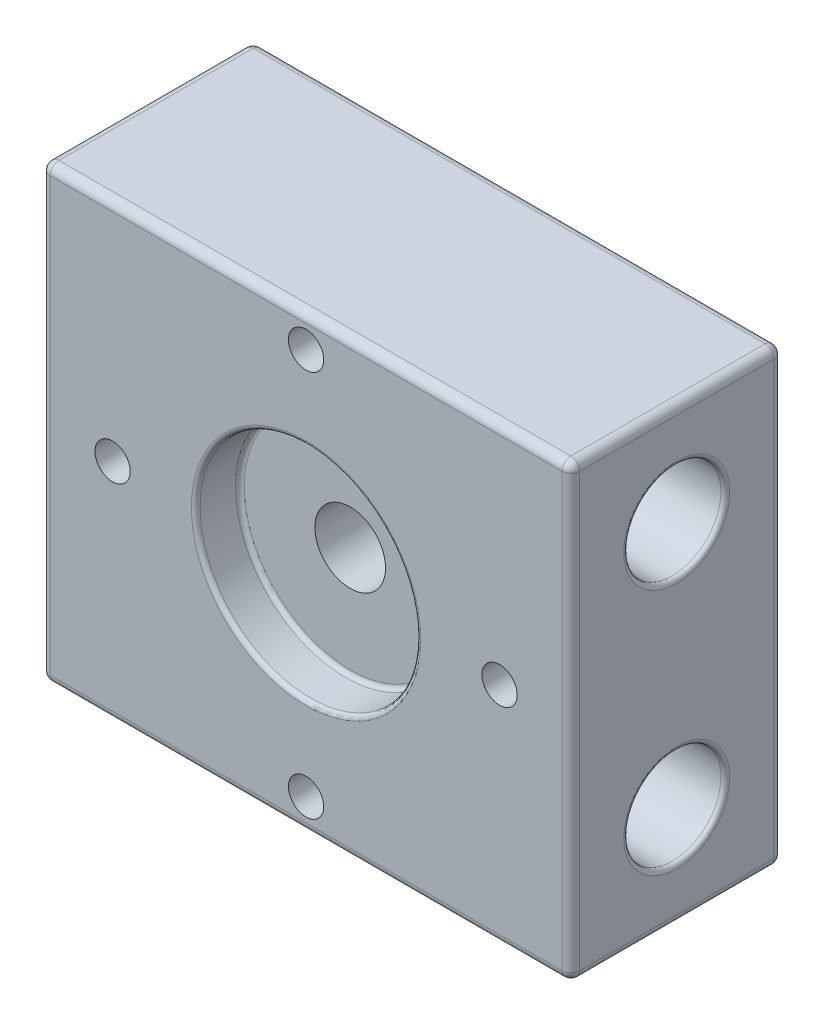
SolidWorks part; units mm, degrees
material "ABS PC"
ref_plane "Front Plane" through (0, 0, 0) normal (0, 0, 1) x (1, 0, 0)
ref_plane "Top Plane" through (0, 0, 0) normal (0, 1, 0) x (1, 0, 0)
ref_plane "Right Plane" through (0, 0, 0) normal (1, 0, 0) x (0, 0, -1)
sketch "Sketch1" plane through (0, 0, 0) normal (0, 0, 1) x (1, 0, 0)
  line L1 (30, -25.5) -> (-30, -25.5)
  line L2 (30, -25.5) -> (30, 25.5)
  line L3 (30, 25.5) -> (-30, 25.5)
  line L4 (-30, -25.5) -> (-30, 25.5)
  line L5 (30, -25.5) -> (-30, 25.5) construction
  line L6 (30, 25.5) -> (-30, -25.5) construction
  point P0 (0, 0)
  dimension "D1" = 60
  dimension "D2" = 51
extrude "Boss-Extrude1" add sketch "Sketch1" along normal mid plane 24
sketch "Sketch2" plane through (0, 0, 12) normal (0, 0, 1) x (1, 0, 0)
  circle A0 centre (0, 0) radius 12.5
  dimension "D1" = 25
extrude "Cut-Extrude1" cut sketch "Sketch2" against normal blind 5
sketch "Sketch3" plane through (30, 0, 0) normal (1, 0, 0) x (0, 0, -1)
  line L0 (0, 0) -> (17.8239, 0) construction
  circle A0 centre (0, 14) radius 5.5
  circle A1 centre (0, -14) radius 5.5
  dimension "D1" = 28
  dimension "D2" = 11
extrude "Cut-Extrude2" cut sketch "Sketch3" against normal through all
fillet "Fillet1" radius 1 12 edges at (-30, -25.5, 0) (0, -25.5, 12) (30, -25.5, 0) (0, -25.5, -12) (30, 25.5, 0) (0, 25.5, 12) (-30, 25.5, 0) (0, 25.5, -12) (-30, 0, -12) (30, 0, -12) (-30, 0, 12) (30, 0, 12)
fillet "Fillet2" radius 0.5 6 edges at (12.5, 0, 12) (12.5, 0, 7) (30, -14, -5.5) (-30, -14, -5.5) (30, 14, -5.5) (-30, 14, -5.5)
sketch "Sketch4" plane through (0, 0, -12) normal (0, 0, -1) x (-1, 0, 0)
  circle A0 centre (0, 0) radius 12.5
  circle A1 centre (0, 0) radius 4
  circle A2 centre (0, 0) radius 12 construction
  dimension "D1" = 25
  dimension "D2" = 8
extrude "Cut-Extrude3" cut sketch "Sketch4" against normal through all contours A1
sketch "Sketch5" plane through (0, 0, -12) normal (0, 0, -1) x (-1, 0, 0)
  line L0 (0, -21.9203) -> (0, 21.9203) construction
  line L1 (-21.9203, 0) -> (21.9203, 0) construction
  circle A4 centre (0, -21.9203) radius 2
  circle A5 centre (-21.9203, 0) radius 2
  circle A6 centre (0, 21.9203) radius 2
  circle A7 centre (21.9203, 0) radius 2
  dimension "D1" = 4
  dimension "D2" = 31
  dimension "D3" = 0
extrude "Cut-Extrude5" cut sketch "Sketch5" against normal through all
